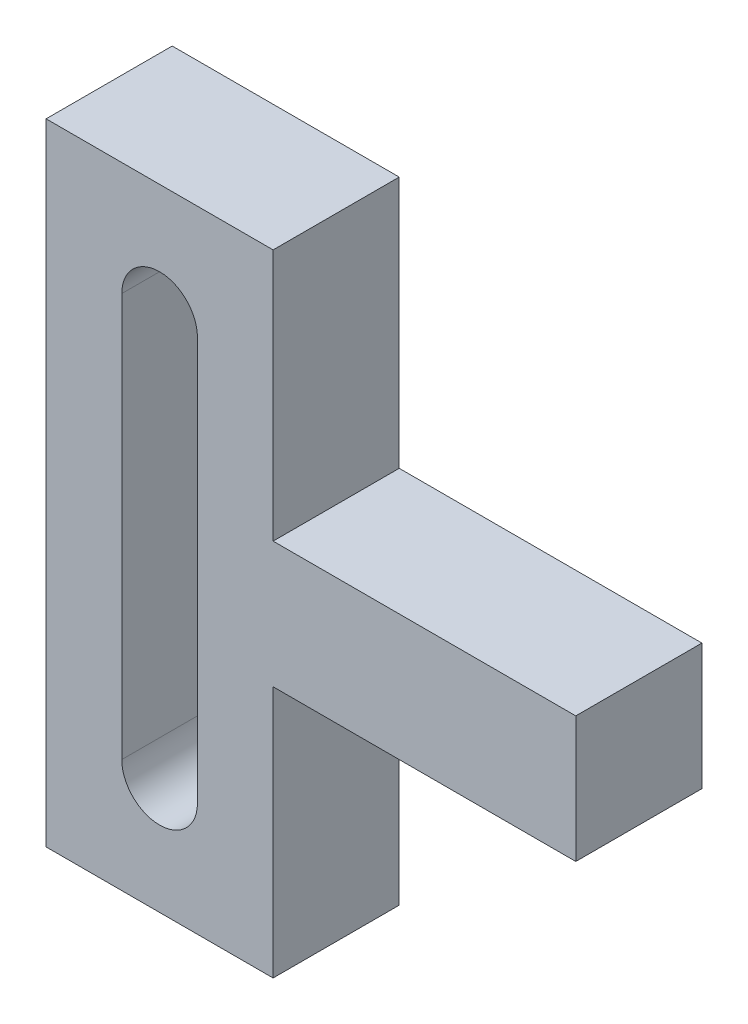
SolidWorks part; units mm, degrees
ref_plane "前视基准面" through (0, 0, 0) normal (0, 0, 1) x (1, 0, 0)
ref_plane "上视基准面" through (0, 0, 0) normal (0, 1, 0) x (1, 0, 0)
ref_plane "右视基准面" through (0, 0, 0) normal (1, 0, 0) x (0, 0, -1)
sketch "草图1" plane through (0, 0, 0) normal (0, 0, 1) x (1, 0, 0)
  line L0 (0, 0) -> (0, 2.5)
  line L1 (0, 2.5) -> (-12, 2.5)
  line L2 (-12, 2.5) -> (-12, 12.5)
  line L3 (-12, 12.5) -> (-21, 12.5)
  line L4 (-21, 12.5) -> (-21, -12.5)
  line L5 (-21, -12.5) -> (-12, -12.5)
  line L6 (-12, -12.5) -> (-12, -2.5)
  line L7 (-12, -2.5) -> (0, -2.5)
  line L8 (0, -2.5) -> (0, 0)
  line L9 (-16.5, -8) -> (-16.5, 8) construction
  line L10 (-18, -8) -> (-18, 8)
  line L11 (-15, -8) -> (-15, 8)
  arc A0 (-18, -8) -> (-15, -8) centre (-16.5, -8) ccw
  arc A1 (-15, 8) -> (-18, 8) centre (-16.5, 8) ccw
  point P12 (-16.5, 0)
  dimension "D5" = 1.5
  dimension "D1" = 5
  dimension "D2" = 12
  dimension "D3" = 9
  dimension "D4" = 10
  dimension "D6" = 16
  dimension "D7" = 3
extrude "凸台-拉伸1" add sketch "草图1" along normal mid plane 5
